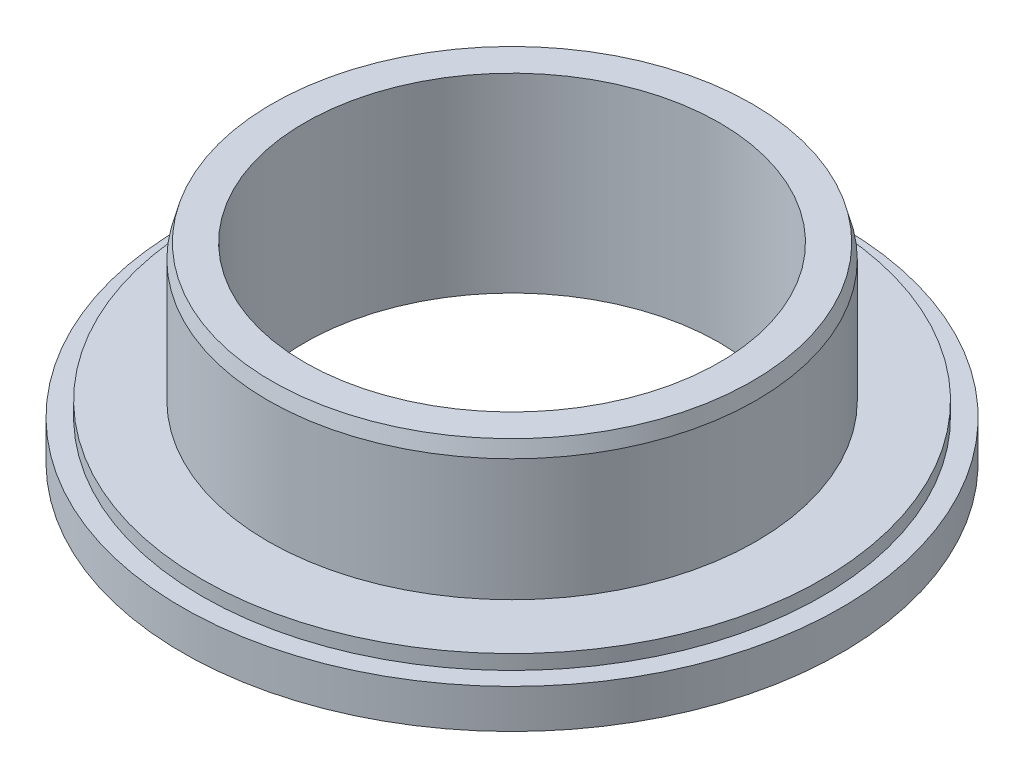
SolidWorks part; units mm, degrees
material "Q235"
ref_plane "Front Plane" through (0, 0, 0) normal (0, 0, 1) x (1, 0, 0)
ref_plane "Top Plane" through (0, 0, 0) normal (0, 1, 0) x (1, 0, 0)
ref_plane "Right Plane" through (0, 0, 0) normal (1, 0, 0) x (0, 0, -1)
sketch "Sketch1" plane through (0, 0, 0) normal (0, 0, 1) x (1, 0, 0)
  line L0 (42.5, 31) -> (50, 31)
  line L1 (50, 31) -> (50, 3)
  line L2 (50, 3) -> (63.5, 3)
  line L3 (63.5, 3) -> (63.5, 0)
  line L4 (63.5, 0) -> (67.5, 0)
  line L5 (67.5, 0) -> (67.5, -8)
  line L6 (67.5, -8) -> (42.5, -8)
  line L7 (42.5, -8) -> (42.5, 31)
  line L8 (0, 0) -> (0, 41.1083) construction
  dimension "D1" = 50
  dimension "D2" = 63.5
  dimension "D3" = 67.5
  dimension "D4" = 28
  dimension "D5" = 3
  dimension "D6" = 8
  dimension "D7" = 42.5
revolve "Revolve1" add sketch "Sketch1" angle 360 about L8
chamfer "Chamfer1" distance 3 angle 15 1 edges at (0, 31, -50)
